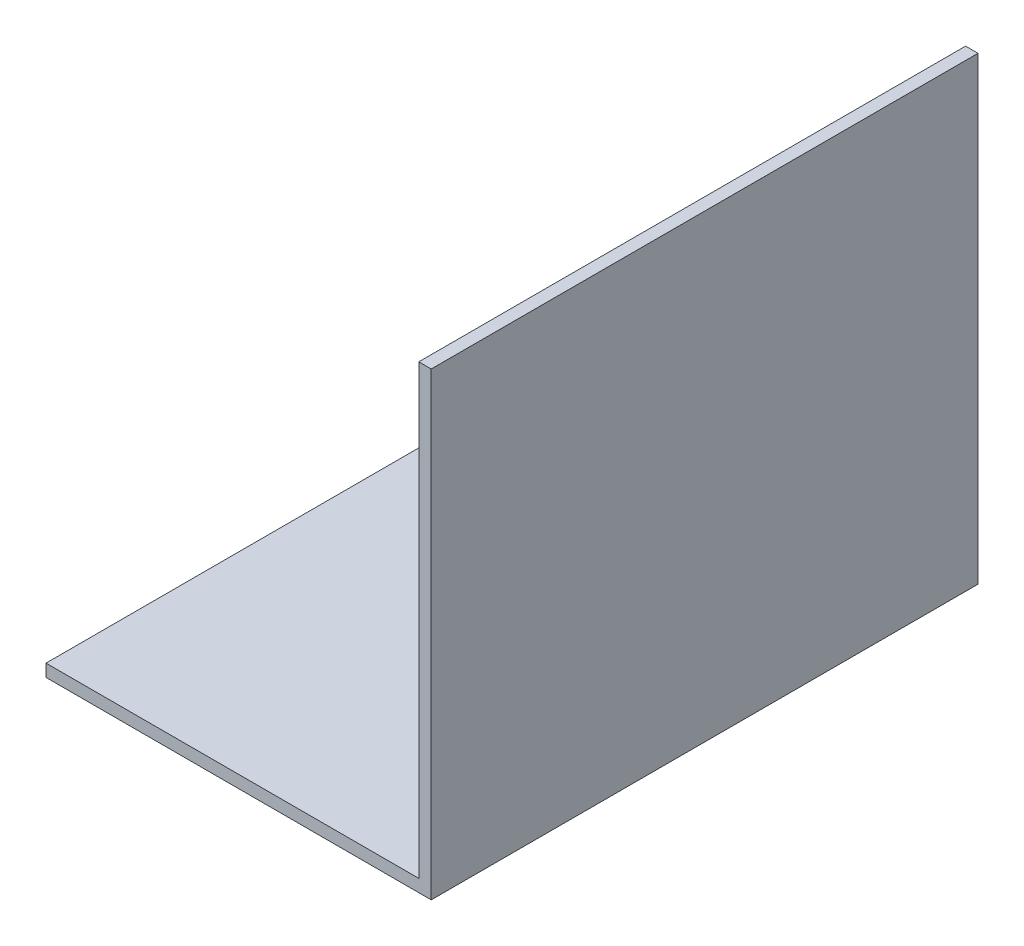
from build123d import *

# Parameters (mm, degrees)
EXTRUDE_1_DEPTH = 110


with BuildPart() as part:
    # 草图1 → 凸台-拉伸1 (new, symmetric)
    with BuildSketch(Plane.XY):
        Polygon((-155, 0), (0, 0), (0, 185), (-5, 185), (-5, 5), (-155, 5), align=None)
    extrude(amount=EXTRUDE_1_DEPTH, both=True)


solid = part.part
